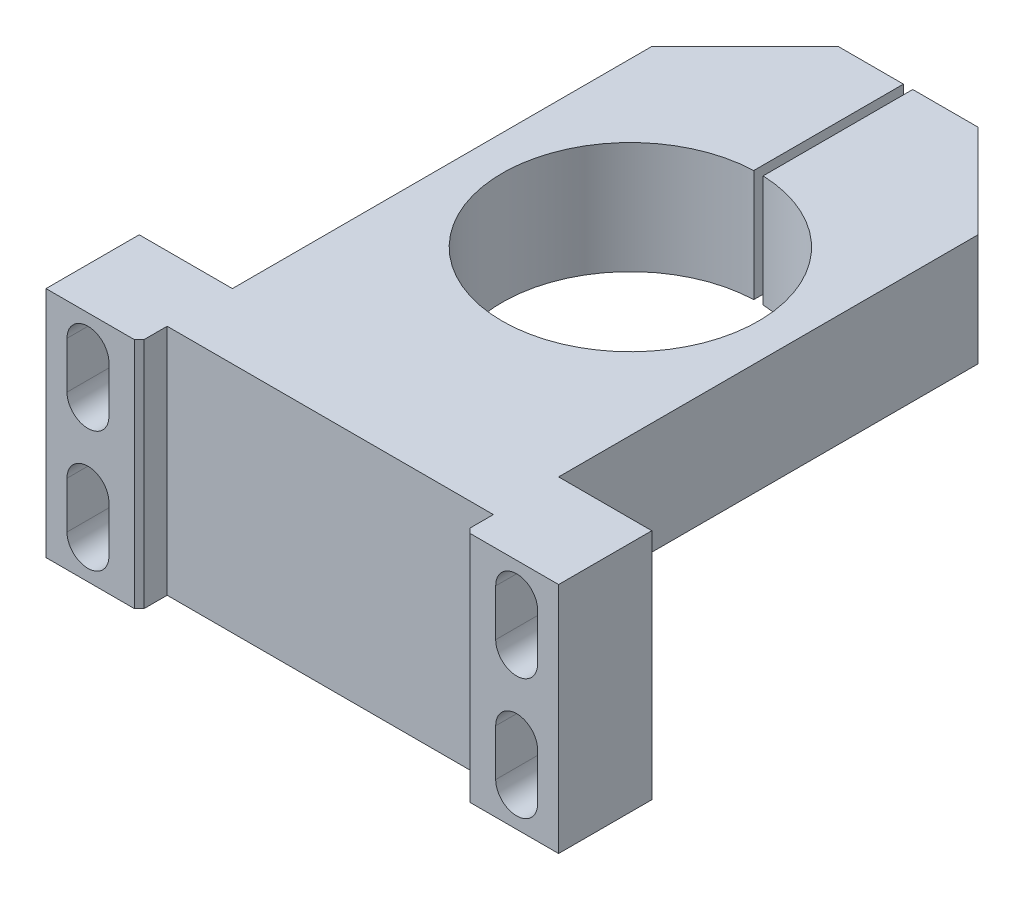
SolidWorks part; units mm, degrees
ref_plane "Front Plane" through (0, 0, 0) normal (0, 0, 1) x (1, 0, 0)
ref_plane "Top Plane" through (0, 0, 0) normal (0, 1, 0) x (1, 0, 0)
ref_plane "Right Plane" through (0, 0, 0) normal (1, 0, 0) x (0, 0, -1)
sketch "Sketch1" plane through (0, 0, 0) normal (0, 1, 0) x (1, 0, 0)
  line L0 (0, 0) -> (0, -50000) construction
  line L2 (-17.5, -35.2) -> (17.5, -35.2)
  line L3 (-17.5, -35.2) -> (-17.5, 29.8)
  line L4 (-17.5, 29.8) -> (17.5, 29.8)
  line L5 (17.5, -35.2) -> (17.5, 29.8)
  line L6 (-17.5, -35.2) -> (17.5, 29.8) construction
  line L7 (-17.5, 29.8) -> (17.5, -35.2) construction
  circle A0 centre (0, 0) radius 13.75
  point P3 (0, -2.7)
  dimension "D1" = 27.5
  dimension "D3" = 35.2
  dimension "D2" = 35
  dimension "D4" = 65
extrude "Boss-Extrude1" add sketch "Sketch1" along normal blind 12
chamfer "Chamfer1" distance 10 angle 45 2 edges at (17.5, 6, -29.8) (-17.5, 6, -29.8)
sketch "Sketch2" plane through (0, 12, 0) normal (0, 1, 0) x (1, 0, 0)
  line L0 (0, 0) -> (0, -50000) construction
  line L1 (-17.5, -35.2) -> (17.5, -35.2) construction
  line L2 (-27.5, -25.2) -> (27.5, -25.2)
  line L3 (-27.5, -25.2) -> (-27.5, -35.2)
  line L4 (-27.5, -35.2) -> (27.5, -35.2)
  line L5 (27.5, -25.2) -> (27.5, -35.2)
  line L6 (-27.5, -25.2) -> (27.5, -35.2) construction
  line L7 (-27.5, -35.2) -> (27.5, -25.2) construction
  point P3 (0, -30.2)
  dimension "D1" = 55
  dimension "D2" = 10
extrude "Boss-Extrude2" add sketch "Sketch2" against normal blind 25
sketch "Sketch3" plane through (0, -13, 0) normal (0, -1, 0) x (1, 0, 0)
  line L0 (0, 0) -> (0, 50000) construction
  line L1 (-27.5, 35.2) -> (27.5, 35.2) construction
  line L2 (-17.5, 38.2) -> (17.5, 38.2)
  line L3 (-17.5, 38.2) -> (-17.5, 32.2)
  line L4 (-17.5, 32.2) -> (17.5, 32.2)
  line L5 (17.5, 38.2) -> (17.5, 32.2)
  line L6 (-17.5, 38.2) -> (17.5, 32.2) construction
  line L7 (-17.5, 32.2) -> (17.5, 38.2) construction
  line L8 (-17.5, -19.8) -> (-17.5, 25.2) construction
  point P3 (0, 35.2)
  dimension "D1" = 3
extrude "Cut-Extrude1" cut sketch "Sketch3" against normal through all
sketch "Sketch4" plane through (0, 0, 25.2) normal (0, 0, -1) x (-1, 0, 0)
  line L0 (0, 0) -> (0, -50000) construction
  line L1 (-27.5, -0.5) -> (49972.5, -0.5) construction
  line L2 (-27.5, -13) -> (-27.5, 12) construction
  line L3 (-23, 8.5) -> (-23, 3.5) construction
  line L4 (-20.75, 8.5) -> (-20.75, 3.5)
  line L5 (-25.25, 8.5) -> (-25.25, 3.5)
  line L6 (23, 8.5) -> (23, 3.5) construction
  line L7 (20.75, 8.5) -> (20.75, 3.5)
  line L8 (25.25, 8.5) -> (25.25, 3.5)
  line L9 (-27.5, 12) -> (-17.5, 12) construction
  line L10 (23, -9.5) -> (23, -4.5) construction
  line L11 (20.75, -9.5) -> (20.75, -4.5)
  line L12 (25.25, -9.5) -> (25.25, -4.5)
  line L13 (-23, -9.5) -> (-23, -4.5) construction
  line L14 (-20.75, -9.5) -> (-20.75, -4.5)
  line L15 (-25.25, -9.5) -> (-25.25, -4.5)
  arc A0 (-20.75, 8.5) -> (-25.25, 8.5) centre (-23, 8.5) ccw
  arc A1 (-25.25, 3.5) -> (-20.75, 3.5) centre (-23, 3.5) ccw
  arc A2 (20.75, 8.5) -> (25.25, 8.5) centre (23, 8.5) cw
  arc A3 (25.25, 3.5) -> (20.75, 3.5) centre (23, 3.5) cw
  arc A4 (20.75, -9.5) -> (25.25, -9.5) centre (23, -9.5) ccw
  arc A5 (25.25, -4.5) -> (20.75, -4.5) centre (23, -4.5) ccw
  arc A6 (-20.75, -9.5) -> (-25.25, -9.5) centre (-23, -9.5) cw
  arc A7 (-25.25, -4.5) -> (-20.75, -4.5) centre (-23, -4.5) cw
  point P7 (-27.5, -0.5)
  point P10 (-23, 6)
  point P17 (23, 6)
  point P26 (23, -7)
  point P33 (-23, -7)
  dimension "D1" = 4.5
  dimension "D2" = 5
  dimension "D3" = 46
  dimension "D4" = 6
extrude "Cut-Extrude2" cut sketch "Sketch4" against normal blind 13.5
chamfer "Chamfer2" distance 0.5 angle 45 2 edges at (17.5, -0.5, 35.2) (-17.5, -0.5, 35.2)
sketch "Sketch5" plane through (0, 12, 0) normal (0, 1, 0) x (1, 0, 0)
  line L0 (0, 0) -> (0, 50000) construction
  line L1 (7.5, 29.8) -> (-7.5, 29.8) construction
  line L2 (-0.5, 48.692) -> (0.5, 48.692)
  line L3 (-0.5, 48.692) -> (-0.5, 10.908)
  line L4 (-0.5, 10.908) -> (0.5, 10.908)
  line L5 (0.5, 48.692) -> (0.5, 10.908)
  line L6 (-0.5, 48.692) -> (0.5, 10.908) construction
  line L7 (-0.5, 10.908) -> (0.5, 48.692) construction
  point P3 (0, 29.8)
  dimension "D1" = 1
extrude "Cut-Extrude3" cut sketch "Sketch5" against normal through all
sketch "Sketch6" plane through (-17.5, 0, 0) normal (-1, 0, 0) x (0, 0, 1)
  line L0 (-29.8, 6) -> (49970.2, 6) construction
  line L1 (-29.8, 0) -> (-29.8, 12) construction
  circle A0 centre (-21.8, 6) radius 5
  point P4 (-29.8, 6)
  dimension "D1" = 10
  dimension "D2" = 8
extrude "Cut-Extrude4" cut sketch "Sketch6" against normal blind 10
sketch "Sketch7" plane through (-7.5, 0, 0) normal (-1, 0, 0) x (0, 0, 1)
  circle A0 centre (-21.8, 6) radius 2.25
  dimension "D1" = 4.5
extrude "Cut-Extrude5" cut sketch "Sketch7" against normal up to surface (7 mm away) up to face at (-0.5, 6, -21.7705)
hole_wizard "M4 Tapped Hole1" positions "Sketch9" profile "Sketch8" tap size "M4" standard "Gb" end condition through all
sketch "Sketch9" plane through (0.5, 0, 0) normal (-1, 0, 0) x (0, 0, 1)
  point P0 (-21.8, 6)
cosmetic thread "Hole thread1" parameters "D2"=4
sketch "Sketch8" plane through (0.5, 6, -21.8) normal (0, 1, 0) x (0, 0, 1)
  line L0 (0, 0) -> (0, 27)
  line L1 (0, 27) -> (1.65, 27)
  line L2 (1.65, 27) -> (1.65, 0)
  line L5 (1.65, 0) -> (0, 0)
  line L11 (0, -6.35) -> (0, 107.95) construction
  dimension "通孔螺纹孔钻头直径" = 3.3
  dimension "通孔螺纹孔钻头深度" = 27
